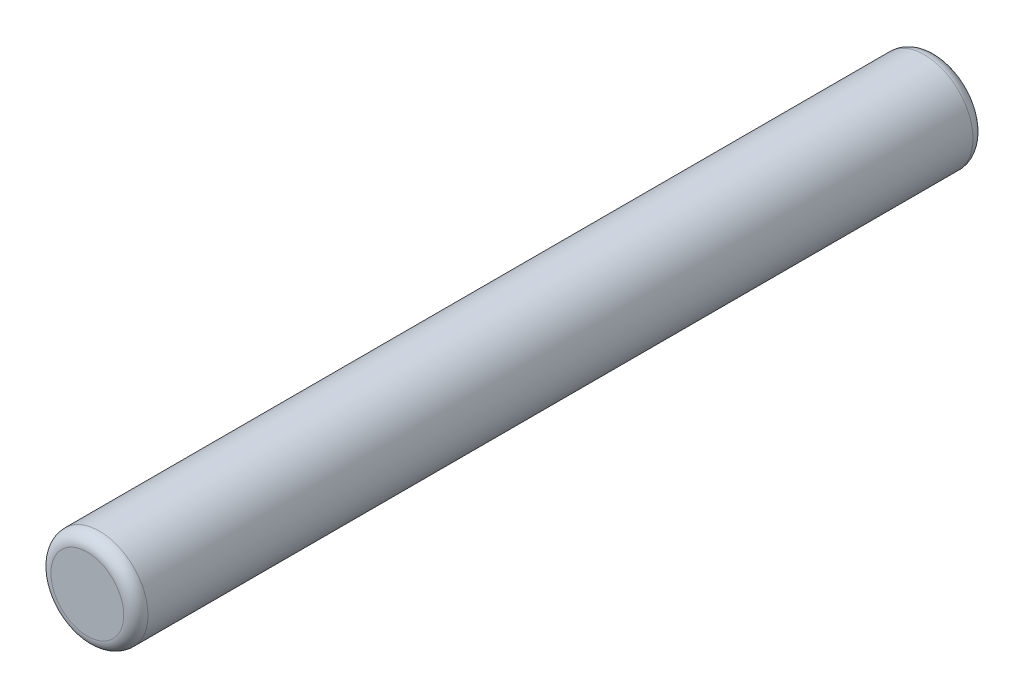
SolidWorks part; units mm, degrees
ref_plane "Front Plane" through (0, 0, 0) normal (0, 0, 1) x (1, 0, 0)
ref_plane "Top Plane" through (0, 0, 0) normal (0, 1, 0) x (1, 0, 0)
ref_plane "Right Plane" through (0, 0, 0) normal (1, 0, 0) x (0, 0, -1)
other "Configuration Table"
sketch "Sketch1" plane through (0, 0, 0) normal (0, 0, 1) x (1, 0, 0)
  circle A0 centre (0, 0) radius 2
  dimension "D1" = 4
extrude "Boss-Extrude1" add sketch "Sketch1" along normal blind 35
fillet "Fillet1" radius 0.5 2 edges at (2, 0, 35) (2, 0, 0)
